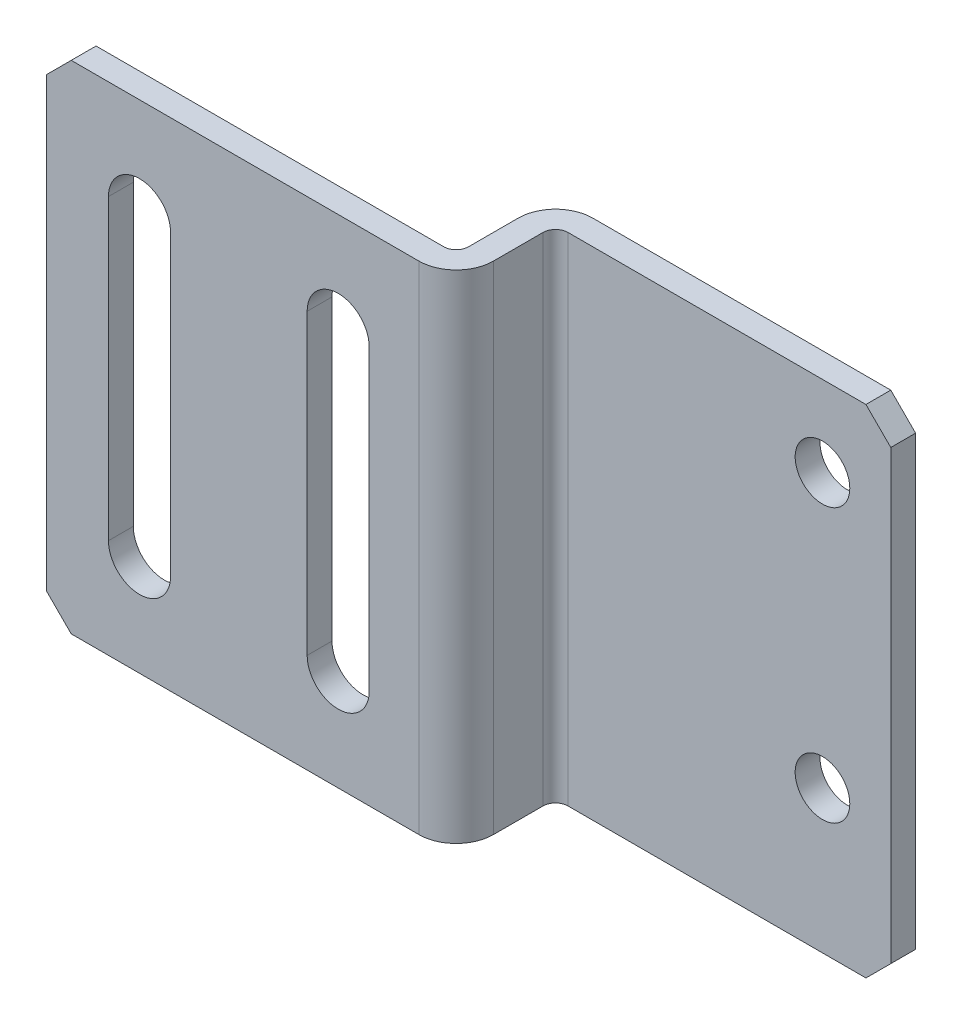
from build123d import *

# Parameters (mm, degrees)
BOSS_EXTRUDE1_DEPTH            = 20
CUT_EXTRUDE1_DEPTH             = 10
CHAMFER1_SIZE                  = 1
FILLET1_R                      = 1.5
FILLET2_R                      = 0.5
F_2_2_2_2_DIAMETER_HOLE1_D     = 2.2
F_2_2_2_2_DIAMETER_HOLE1_DEPTH = 5
F_2_2_2_2_DIAMETER_HOLE1_TIP   = 0.660946681


with BuildPart() as part:
    # Sketch1 → Boss-Extrude1 (new body)
    with BuildSketch(Plane(origin=(0, 0, 0), x_dir=(1, 0, 0), z_dir=(0, 1, 0))):
        Polygon((0, 0), (16.5, 0), (16.5, 4), (30, 4), (30, 5), (15.5, 5), (15.5, 1), (0, 1), align=None)
    extrude(amount=BOSS_EXTRUDE1_DEPTH)

    # Sketch2 → Cut-Extrude1 (cut)
    with BuildSketch(Plane(origin=(0, 0, -5), x_dir=(-1, 0, 0), z_dir=(0, 0, -1))):
        with BuildLine():
            Line((-10.5, 16), (-10.5, 4))
            ThreePointArc((-10.5, 4), (-11.75, 2.75), (-13, 4))
            Line((-13, 4), (-13, 16))
            ThreePointArc((-13, 16), (-11.75, 17.25), (-10.5, 16))
        make_face()
        with BuildLine():
            Line((-5, 16), (-5, 4))
            ThreePointArc((-5, 4), (-3.75, 2.75), (-2.5, 4))
            Line((-2.5, 4), (-2.5, 16))
            ThreePointArc((-2.5, 16), (-3.75, 17.25), (-5, 16))
        make_face()
    extrude(amount=-CUT_EXTRUDE1_DEPTH, mode=Mode.SUBTRACT)

    # Chamfer1
    chamfer1_edges = [part.edges().sort_by_distance(p)[0] for p in [
        (0, 0, -0.5),
        (30, 20, -4.5),
        (0, 20, -0.5),
        (30, 0, -4.5),
    ]]
    chamfer(chamfer1_edges, length=CHAMFER1_SIZE)

    # Fillet1
    fillet1_edges = [part.edges().sort_by_distance(p)[0] for p in [
        (15.5, 10, -5),
        (16.5, 10, 0),
    ]]
    fillet(fillet1_edges, radius=FILLET1_R)

    # Fillet2
    fillet2_edges = [part.edges().sort_by_distance(p)[0] for p in [
        (15.5, 10, -1),
        (16.5, 10, -4),
    ]]
    fillet(fillet2_edges, radius=FILLET2_R)

    # Ø2.2 (2.2) Diameter Hole1
    with Locations(Plane.XY.offset(-4)):
        with Locations((27.25, 16.75), (27.25, 5.75)):
            Hole(F_2_2_2_2_DIAMETER_HOLE1_D / 2, depth=F_2_2_2_2_DIAMETER_HOLE1_DEPTH)
            with Locations((0, 0, -(F_2_2_2_2_DIAMETER_HOLE1_DEPTH + F_2_2_2_2_DIAMETER_HOLE1_TIP / 2))):  # 118° drill point
                Cone(0, F_2_2_2_2_DIAMETER_HOLE1_D / 2, F_2_2_2_2_DIAMETER_HOLE1_TIP, mode=Mode.SUBTRACT)


solid = part.part
